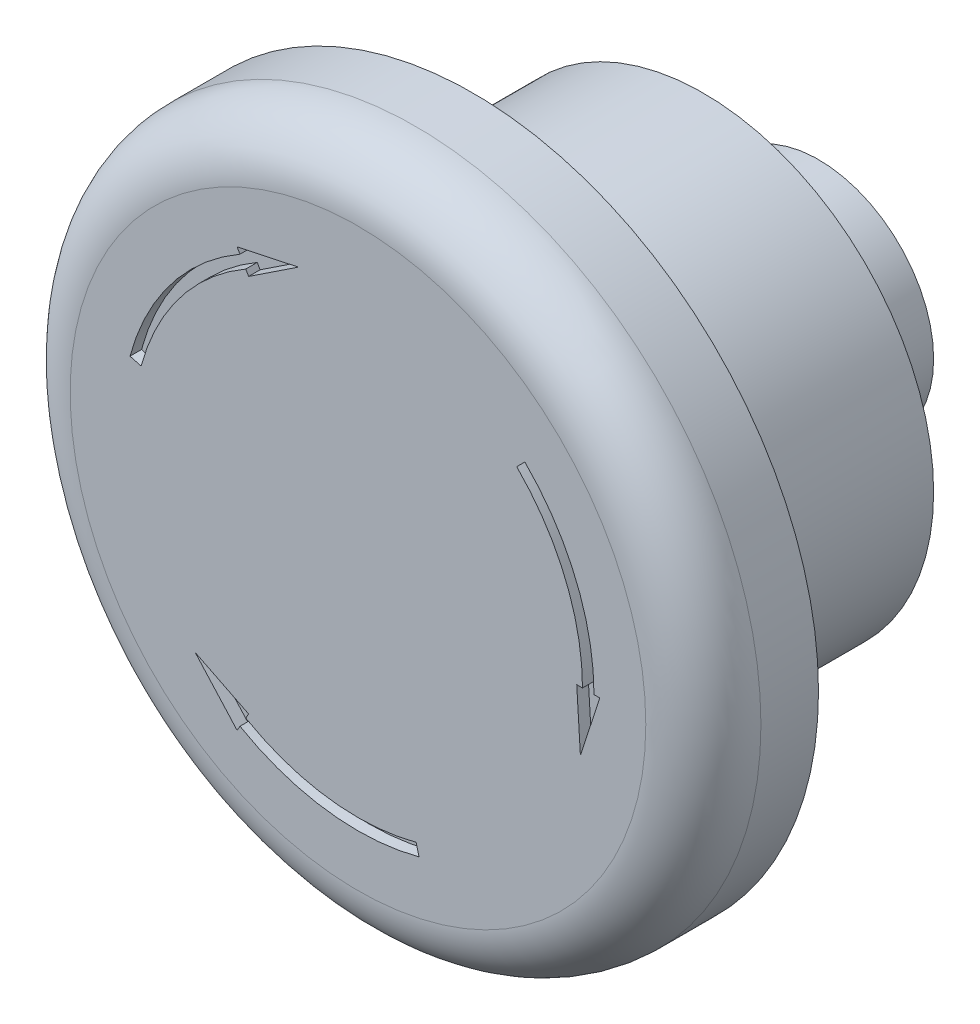
SolidWorks part; units mm, degrees
ref_plane "前视基准面" through (0, 0, 0) normal (0, 0, 1) x (1, 0, 0)
ref_plane "上视基准面" through (0, 0, 0) normal (0, 1, 0) x (1, 0, 0)
ref_plane "右视基准面" through (0, 0, 0) normal (1, 0, 0) x (0, 0, -1)
sketch "草图1" plane through (0, 0, 0) normal (0, 0, 1) x (1, 0, 0)
  circle A0 centre (0, 0) radius 100
extrude "凸台-拉伸1" add sketch "草图1" along normal blind 100
sketch "草图2" plane through (0, 0, 100) normal (0, 0, 1) x (1, 0, 0)
  circle A0 centre (0, 0) radius 200
extrude "凸台-拉伸2" add sketch "草图2" along normal blind 200
sketch "草图3" plane through (0, 0, 300) normal (0, 0, 1) x (1, 0, 0)
  circle A0 centre (0, 0) radius 300
extrude "凸台-拉伸3" add sketch "草图3" along normal blind 100 contours A0
sketch "草图4" plane through (0, 0, 400) normal (0, 0, 1) x (1, 0, 0)
  line L3 (-188.3555, 50.4697) -> (-198.0148, 53.0579)
  line L9 (-105, 181.8653) -> (-102.5, 177.5352)
  line L10 (-97.5, 168.875) -> (-95, 164.5448)
  line L12 (-105, 181.8653) -> (-51.7638, 193.1852)
  line L14 (-95, 164.5448) -> (-51.7638, 193.1852)
  arc A0 (-102.5, 177.5352) -> (-198.0148, 53.0579) centre (0, 0) ccw
  arc A3 (-97.5, 168.875) -> (-188.3555, 50.4697) centre (0, 0) ccw
extrude "切除-拉伸1" cut sketch "草图4" against normal blind 10
pattern_circular "阵列(圆周)1" count 3 over 360 about axis through (0, 0, 0) along (0, 0, 1) of "切除-拉伸1"
fillet "圆角1" radius 50 1 edges at (300, 0, 400)
scale "缩放比例1" scale about centroid uniform scaling yes scale factor 0.1
